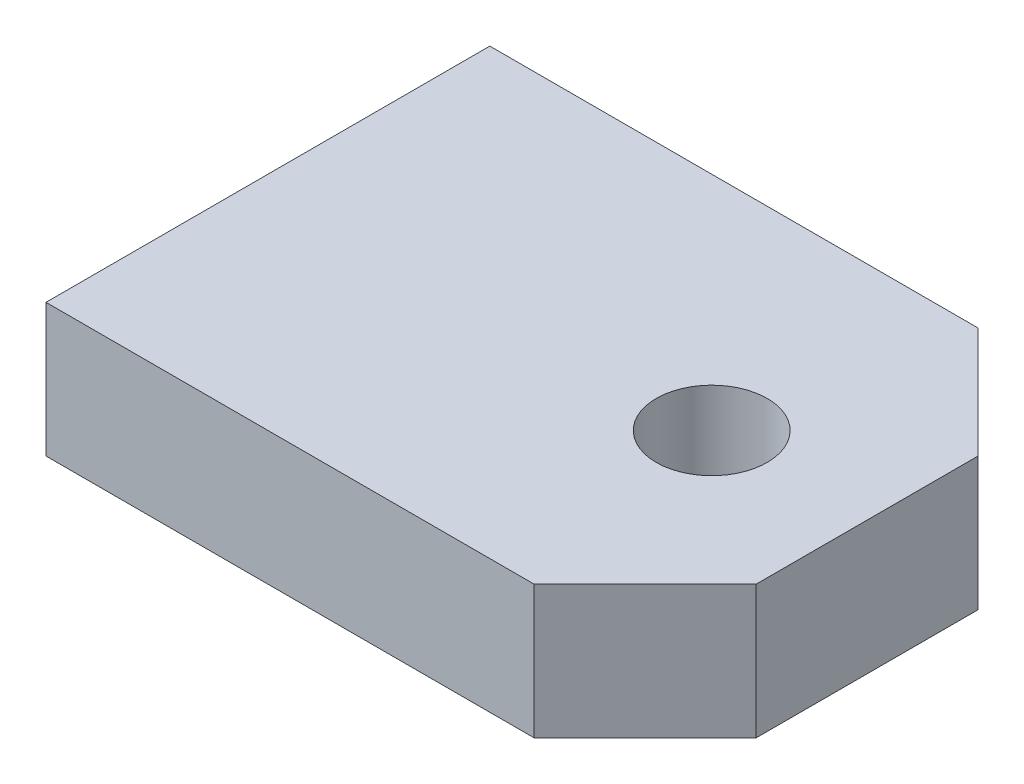
SolidWorks part; units mm, degrees
material "1023 碳钢板 (SS)"
ref_plane "前视基准面" through (0, 0, 0) normal (0, 0, 1) x (1, 0, 0)
ref_plane "上视基准面" through (0, 0, 0) normal (0, 1, 0) x (1, 0, 0)
ref_plane "右视基准面" through (0, 0, 0) normal (1, 0, 0) x (0, 0, -1)
sketch "草图1" plane through (0, 0, 0) normal (0, 0, 1) x (1, 0, 0)
  line L1 (-13.5, 3) -> (13.5, 3)
  line L2 (-13.5, 3) -> (-13.5, -3)
  line L3 (-13.5, -3) -> (13.5, -3)
  line L4 (13.5, 3) -> (13.5, -3)
  line L5 (-13.5, 3) -> (13.5, -3) construction
  line L6 (-13.5, -3) -> (13.5, 3) construction
  point P0 (0, 0)
  dimension "D1" = 27
  dimension "D2" = 6
extrude "凸台-拉伸1" add sketch "草图1" along normal blind 20
sketch "草图2" plane through (0, 3, 0) normal (0, 1, 0) x (1, 0, 0)
  line L0 (13.5, -20) -> (13.5, 0) construction
  circle A0 centre (6.5, -10) radius 2.0313
  dimension "D1" = 7
hole_wizard "M6 螺纹孔1" positions "草图3" profile "草图4" tap size "M6" standard "GB"
sketch "草图3" plane through (0, 3, 0) normal (0, 1, 0) x (1, 0, 0)
  point P0 (6.5, -10)
sketch "草图4" plane through (6.5, 3, 10) normal (1, 0, 0) x (0, 0, 1)
  line L0 (0, 0) -> (0, 16.5022)
  line L1 (0, 16.5022) -> (2.5, 15)
  line L2 (2.5, 15) -> (2.5, 0)
  line L5 (2.5, 0) -> (0, 0)
  line L10 (0, 16.5022) -> (-2.5, 15) construction
  line L11 (0, -6.35) -> (0, 107.95) construction
  dimension "螺纹孔钻头直径" = 5
  dimension "螺纹孔钻头深度" = 15
  dimension "导头角度" = 118
cosmetic thread "孔螺蚊线1" parameters "D1"=12, "D2"=6
chamfer "倒角1" distance 5 angle 45 2 edges at (13.5, 0, 0) (13.5, 0, 20)
